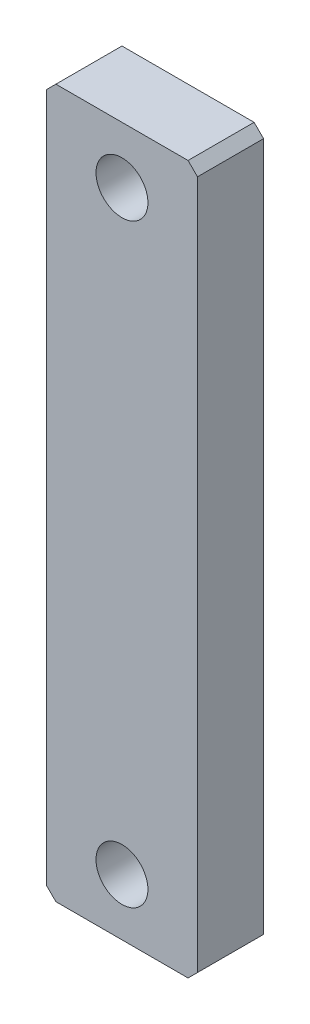
SolidWorks part; units mm, degrees
material "45"
ref_plane "Front Plane" through (0, 0, 0) normal (0, 0, 1) x (1, 0, 0)
ref_plane "Top Plane" through (0, 0, 0) normal (0, 1, 0) x (1, 0, 0)
ref_plane "Right Plane" through (0, 0, 0) normal (1, 0, 0) x (0, 0, -1)
sketch "Sketch1" plane through (0, 0, 0) normal (0, 0, 1) x (1, 0, 0)
  line L1 (-8, 37.5) -> (8, 37.5)
  line L2 (-8, 37.5) -> (-8, -37.5)
  line L3 (-8, -37.5) -> (8, -37.5)
  line L4 (8, 37.5) -> (8, -37.5)
  line L5 (-8, 37.5) -> (8, -37.5) construction
  line L6 (-8, -37.5) -> (8, 37.5) construction
  point P0 (0, 0)
  dimension "D1" = 16
  dimension "D2" = 75
extrude "Boss-Extrude1" add sketch "Sketch1" along normal blind 7
chamfer "Chamfer5" distance 1 angle 45 4 edges at (8, 37.5, 3.5) (8, -37.5, 3.5) (-8, -37.5, 3.5) (-8, 37.5, 3.5)
hole_wizard "M5 Clearance Hole1" positions "Sketch14" profile "Sketch15" hole size "M5" standard "GB" end condition through all
sketch "Sketch14" plane through (0, 0, 7) normal (0, 0, 1) x (1, 0, 0)
  line L0 (-41.0032, 0) -> (42.7091, 0) construction
  line L2 (-8, 36.5) -> (-8, -36.5) construction
  line L3 (-7, -37.5) -> (7, -37.5) construction
  point P0 (0, 31.5)
  point P4 (0, -31.5)
  dimension "D1" = 8
  dimension "D3" = 6
sketch "Sketch15" plane through (0, 31.5, 7) normal (1, 0, 0) x (0, -1, 0)
  line L0 (0, 0) -> (0, 7)
  line L1 (0, 7) -> (2.75, 7)
  line L2 (2.75, 7) -> (2.75, 0)
  line L5 (2.75, 0) -> (0, 0)
  line L11 (0, -6.35) -> (0, 107.95) construction
  dimension "通孔孔直径" = 5.5
  dimension "通孔孔深度" = 7
